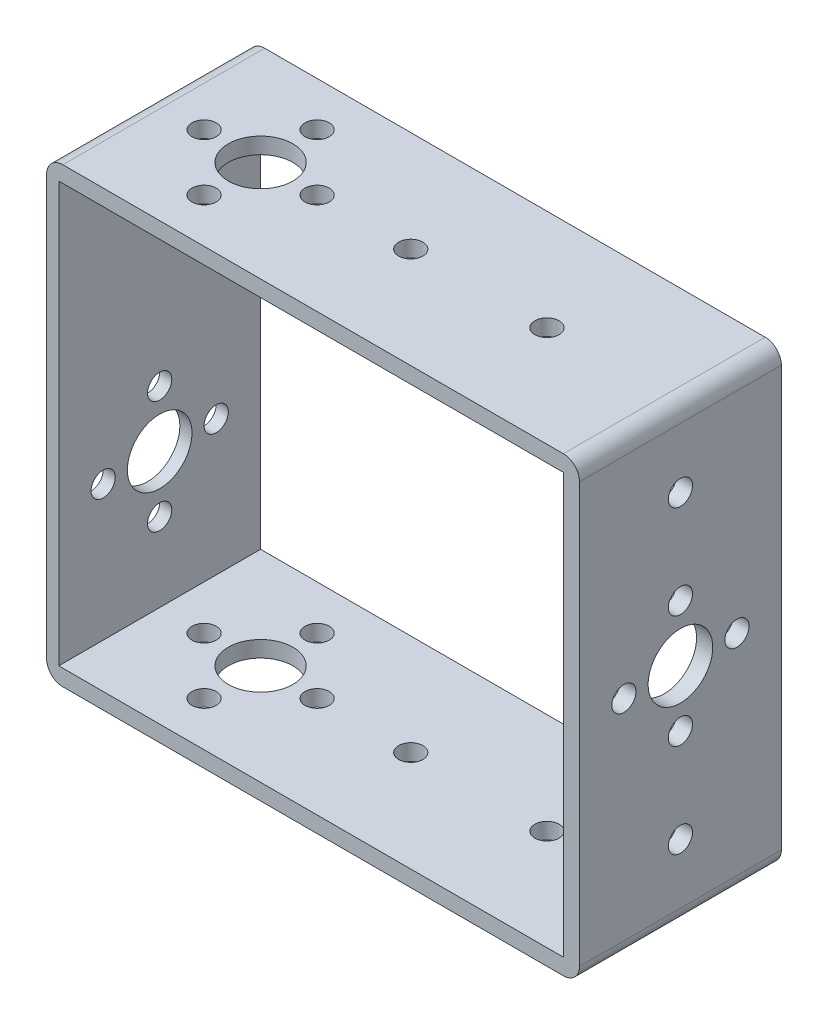
from build123d import *

# Parameters (mm, degrees)
SKETCH1_W                       = 64.5
SKETCH1_H                       = 56
BOSS_EXTRUDE1_DEPTH             = 25
CUT_EXTRUDE1_REACH              = 51.488
SKETCH2_W                       = 62.5
SKETCH2_H                       = 52
CUT_EXTRUDE2_REACH              = 76.627
SKETCH3_R                       = 4
SKETCH3_R_2                     = 1.5
CUT_EXTRUDE3_REACH              = 71.29
SKETCH4_R                       = 4
SKETCH4_R_2                     = 1.5
FILLET3_R                       = 2
BOSS_EXTRUDE2_REACH             = 51.488
SKETCH5_W                       = 1.5
SKETCH5_H                       = 25
BOSS_EXTRUDE2_DIRECTION_2_REACH = 51.488
FILLET4_R                       = 2
SKETCH6_R                       = 1.5
SKETCH6_R_2                     = 4
CUT_EXTRUDE5_DEPTH              = 1.5


with BuildPart() as part:
    # Sketch1 → Boss-Extrude1 (new body)
    with BuildSketch(Plane.XY):
        Rectangle(SKETCH1_W, SKETCH1_H)
    extrude(amount=BOSS_EXTRUDE1_DEPTH)

    # Sketch2 → Cut-Extrude1 (cut, up to next)
    with BuildSketch(Plane.XY.offset(25), mode=Mode.PRIVATE) as cut_extrude1_sk1:
        with Locations((-1, 0)):
            Rectangle(SKETCH2_W, SKETCH2_H)
    cut_extrude1_tool1 = extrude(cut_extrude1_sk1.sketch, amount=-CUT_EXTRUDE1_REACH, mode=Mode.PRIVATE) & part.part
    add(cut_extrude1_tool1.solids().sort_by_distance((-1, 0, 25))[0], mode=Mode.SUBTRACT)

    # Sketch3 → Cut-Extrude2 (cut, up to next)
    with BuildSketch(Plane(origin=(32.25, 0, 0), x_dir=(0, 0, -1), z_dir=(1, 0, 0)), mode=Mode.PRIVATE) as cut_extrude2_sk1:
        with Locations((-12.5, 0)):
            Circle(SKETCH3_R)
    cut_extrude2_tool1 = extrude(cut_extrude2_sk1.sketch, amount=-CUT_EXTRUDE2_REACH, mode=Mode.PRIVATE) & part.part
    # Sketch3 → Cut-Extrude2 (cut, up to next)
    with BuildSketch(Plane(origin=(32.25, 0, 0), x_dir=(0, 0, -1), z_dir=(1, 0, 0)), mode=Mode.PRIVATE) as cut_extrude2_sk2:
        with Locations((-5.5, 0)):
            Circle(SKETCH3_R_2)
    cut_extrude2_tool2 = extrude(cut_extrude2_sk2.sketch, amount=-CUT_EXTRUDE2_REACH, mode=Mode.PRIVATE) & part.part
    # Sketch3 → Cut-Extrude2 (cut, up to next)
    with BuildSketch(Plane(origin=(32.25, 0, 0), x_dir=(0, 0, -1), z_dir=(1, 0, 0)), mode=Mode.PRIVATE) as cut_extrude2_sk3:
        with Locations((-12.5, 18.6)):
            Circle(SKETCH3_R_2)
    cut_extrude2_tool3 = extrude(cut_extrude2_sk3.sketch, amount=-CUT_EXTRUDE2_REACH, mode=Mode.PRIVATE) & part.part
    # Sketch3 → Cut-Extrude2 (cut, up to next)
    with BuildSketch(Plane(origin=(32.25, 0, 0), x_dir=(0, 0, -1), z_dir=(1, 0, 0)), mode=Mode.PRIVATE) as cut_extrude2_sk4:
        with Locations((-12.5, -7)):
            Circle(SKETCH3_R_2)
    cut_extrude2_tool4 = extrude(cut_extrude2_sk4.sketch, amount=-CUT_EXTRUDE2_REACH, mode=Mode.PRIVATE) & part.part
    # Sketch3 → Cut-Extrude2 (cut, up to next)
    with BuildSketch(Plane(origin=(32.25, 0, 0), x_dir=(0, 0, -1), z_dir=(1, 0, 0)), mode=Mode.PRIVATE) as cut_extrude2_sk5:
        with Locations((-19.5, 0)):
            Circle(SKETCH3_R_2)
    cut_extrude2_tool5 = extrude(cut_extrude2_sk5.sketch, amount=-CUT_EXTRUDE2_REACH, mode=Mode.PRIVATE) & part.part
    # Sketch3 → Cut-Extrude2 (cut, up to next)
    with BuildSketch(Plane(origin=(32.25, 0, 0), x_dir=(0, 0, -1), z_dir=(1, 0, 0)), mode=Mode.PRIVATE) as cut_extrude2_sk6:
        with Locations((-12.5, 7)):
            Circle(SKETCH3_R_2)
    cut_extrude2_tool6 = extrude(cut_extrude2_sk6.sketch, amount=-CUT_EXTRUDE2_REACH, mode=Mode.PRIVATE) & part.part
    # Sketch3 → Cut-Extrude2 (cut, up to next)
    with BuildSketch(Plane(origin=(32.25, 0, 0), x_dir=(0, 0, -1), z_dir=(1, 0, 0)), mode=Mode.PRIVATE) as cut_extrude2_sk7:
        with Locations(Location((-12.5, -18.6, 0), (0, 0, 90))):
            Circle(SKETCH3_R_2)
    cut_extrude2_tool7 = extrude(cut_extrude2_sk7.sketch, amount=-CUT_EXTRUDE2_REACH, mode=Mode.PRIVATE) & part.part
    add(cut_extrude2_tool1.solids().sort_by_distance((32.25, 0, 12.5))[0], mode=Mode.SUBTRACT)
    add(cut_extrude2_tool2.solids().sort_by_distance((32.25, 0, 5.5))[0], mode=Mode.SUBTRACT)
    add(cut_extrude2_tool3.solids().sort_by_distance((32.25, 18.6, 12.5))[0], mode=Mode.SUBTRACT)
    add(cut_extrude2_tool4.solids().sort_by_distance((32.25, -7, 12.5))[0], mode=Mode.SUBTRACT)
    add(cut_extrude2_tool5.solids().sort_by_distance((32.25, 0, 19.5))[0], mode=Mode.SUBTRACT)
    add(cut_extrude2_tool6.solids().sort_by_distance((32.25, 7, 12.5))[0], mode=Mode.SUBTRACT)
    add(cut_extrude2_tool7.solids().sort_by_distance((32.25, -18.6, 12.5))[0], mode=Mode.SUBTRACT)

    # Sketch4 → Cut-Extrude3 (cut, up to next)
    with BuildSketch(Plane.XZ.offset(28), mode=Mode.PRIVATE) as cut_extrude3_sk1:
        with Locations(Location((-19.75, 12.5, 0), (0, 0, 270))):
            Circle(SKETCH4_R)
    cut_extrude3_tool1 = extrude(cut_extrude3_sk1.sketch, amount=-CUT_EXTRUDE3_REACH, mode=Mode.PRIVATE) & part.part
    # Sketch4 → Cut-Extrude3 (cut, up to next)
    with BuildSketch(Plane.XZ.offset(28), mode=Mode.PRIVATE) as cut_extrude3_sk2:
        with Locations(Location((-12.75, 12.5, 0), (0, 0, 270))):
            Circle(SKETCH4_R_2)
    cut_extrude3_tool2 = extrude(cut_extrude3_sk2.sketch, amount=-CUT_EXTRUDE3_REACH, mode=Mode.PRIVATE) & part.part
    # Sketch4 → Cut-Extrude3 (cut, up to next)
    with BuildSketch(Plane.XZ.offset(28), mode=Mode.PRIVATE) as cut_extrude3_sk3:
        with Locations(Location((-1.15, 12.5, 0), (0, 0, 270))):
            Circle(SKETCH4_R_2)
    cut_extrude3_tool3 = extrude(cut_extrude3_sk3.sketch, amount=-CUT_EXTRUDE3_REACH, mode=Mode.PRIVATE) & part.part
    # Sketch4 → Cut-Extrude3 (cut, up to next)
    with BuildSketch(Plane.XZ.offset(28), mode=Mode.PRIVATE) as cut_extrude3_sk4:
        with Locations(Location((15.72, 12.5, 0), (0, 0, 270))):
            Circle(SKETCH4_R_2)
    cut_extrude3_tool4 = extrude(cut_extrude3_sk4.sketch, amount=-CUT_EXTRUDE3_REACH, mode=Mode.PRIVATE) & part.part
    # Sketch4 → Cut-Extrude3 (cut, up to next)
    with BuildSketch(Plane.XZ.offset(28), mode=Mode.PRIVATE) as cut_extrude3_sk5:
        with Locations(Location((-19.75, 5.5, 0), (0, 0, 270))):
            Circle(SKETCH4_R_2)
    cut_extrude3_tool5 = extrude(cut_extrude3_sk5.sketch, amount=-CUT_EXTRUDE3_REACH, mode=Mode.PRIVATE) & part.part
    # Sketch4 → Cut-Extrude3 (cut, up to next)
    with BuildSketch(Plane.XZ.offset(28), mode=Mode.PRIVATE) as cut_extrude3_sk6:
        with Locations(Location((-26.75, 12.5, 0), (0, 0, 270))):
            Circle(SKETCH4_R_2)
    cut_extrude3_tool6 = extrude(cut_extrude3_sk6.sketch, amount=-CUT_EXTRUDE3_REACH, mode=Mode.PRIVATE) & part.part
    # Sketch4 → Cut-Extrude3 (cut, up to next)
    with BuildSketch(Plane.XZ.offset(28), mode=Mode.PRIVATE) as cut_extrude3_sk7:
        with Locations(Location((-19.75, 19.5, 0), (0, 0, 270))):
            Circle(SKETCH4_R_2)
    cut_extrude3_tool7 = extrude(cut_extrude3_sk7.sketch, amount=-CUT_EXTRUDE3_REACH, mode=Mode.PRIVATE) & part.part
    cut_extrude3_1 = cut_extrude3_tool1.solids().sort_by_distance((-19.75, -28, 12.5))[0]
    add(cut_extrude3_1, mode=Mode.SUBTRACT)
    cut_extrude3_2 = cut_extrude3_tool2.solids().sort_by_distance((-12.75, -28, 12.5))[0]
    add(cut_extrude3_2, mode=Mode.SUBTRACT)
    cut_extrude3_3 = cut_extrude3_tool3.solids().sort_by_distance((-1.15, -28, 12.5))[0]
    add(cut_extrude3_3, mode=Mode.SUBTRACT)
    cut_extrude3_4 = cut_extrude3_tool4.solids().sort_by_distance((15.72, -28, 12.5))[0]
    add(cut_extrude3_4, mode=Mode.SUBTRACT)
    cut_extrude3_5 = cut_extrude3_tool5.solids().sort_by_distance((-19.75, -28, 5.5))[0]
    add(cut_extrude3_5, mode=Mode.SUBTRACT)
    cut_extrude3_6 = cut_extrude3_tool6.solids().sort_by_distance((-26.75, -28, 12.5))[0]
    add(cut_extrude3_6, mode=Mode.SUBTRACT)
    cut_extrude3_7 = cut_extrude3_tool7.solids().sort_by_distance((-19.75, -28, 19.5))[0]
    add(cut_extrude3_7, mode=Mode.SUBTRACT)
    cut_extrude3 = cut_extrude3_1 + cut_extrude3_2 + cut_extrude3_3 + cut_extrude3_4 + cut_extrude3_5 + cut_extrude3_6 + cut_extrude3_7  # Cut-Extrude3 as one shape, for the pattern or mirror that repeats it

    # Mirror1: Cut-Extrude3 across plane
    add(cut_extrude3.mirror(Plane.ZX), mode=Mode.SUBTRACT)

    # Fillet3
    fillet3_edges = [part.edges().sort_by_distance(p)[0] for p in [
        (32.25, -28, 12.5),
        (32.25, 28, 12.5),
    ]]
    fillet(fillet3_edges, radius=FILLET3_R)

    # Boss-Extrude2: up to this face of the body (flat: up to its plane)
    boss_extrude2_end = Plane(part.part.faces().sort_by_distance((-1, 28, 0.673145601))[0])
    # Sketch5 → Boss-Extrude2 (add, up to the picked face)
    with BuildSketch(Plane(origin=(0, 0, 0), x_dir=(1, 0, 0), z_dir=(0, 1, 0)), mode=Mode.PRIVATE) as boss_extrude2_sk1:
        with Locations((-33, -12.5)):
            Rectangle(SKETCH5_W, SKETCH5_H)
    boss_extrude2_tool1 = split(extrude(boss_extrude2_sk1.sketch, amount=BOSS_EXTRUDE2_REACH, mode=Mode.PRIVATE), bisect_by=boss_extrude2_end, keep=Keep.BOTH, mode=Mode.PRIVATE)
    add(boss_extrude2_tool1.solids().sort_by(Axis((-33, 0, 12.5), (0, 1, 0)))[0])

    # Boss-Extrude2 direction 2: up to this face of the body (flat: up to its plane)
    boss_extrude2_direction_2_end = Plane(part.part.faces().sort_by_distance((-1, -28, 0.673145601))[0])
    # Sketch5 → Boss-Extrude2 direction 2 (add, up to the picked face)
    with BuildSketch(Plane(origin=(0, 0, 0), x_dir=(1, 0, 0), z_dir=(0, 1, 0)), mode=Mode.PRIVATE) as boss_extrude2_direction_2_sk1:
        with Locations((-33, -12.5)):
            Rectangle(SKETCH5_W, SKETCH5_H)
    boss_extrude2_direction_2_tool1 = split(extrude(boss_extrude2_direction_2_sk1.sketch, amount=-BOSS_EXTRUDE2_DIRECTION_2_REACH, mode=Mode.PRIVATE), bisect_by=boss_extrude2_direction_2_end, keep=Keep.BOTH, mode=Mode.PRIVATE)
    add(boss_extrude2_direction_2_tool1.solids().sort_by(Axis((-33, 0, 12.5), (0, -1, 0)))[0])

    # Fillet4
    fillet4_edges = [part.edges().sort_by_distance(p)[0] for p in [
        (-33.75, 28, 12.5),
        (-33.75, -28, 12.5),
    ]]
    fillet(fillet4_edges, radius=FILLET4_R)

    # Sketch6 → Cut-Extrude5 (cut)
    with BuildSketch(Plane(origin=(-32.25, 0, 0), x_dir=(0, 0, -1), z_dir=(1, 0, 0))):
        with Locations((-12.5, -2.25)):
            Circle(SKETCH6_R)
        with Locations((-19.5, -9.25)):
            Circle(SKETCH6_R)
        with Locations((-5.5, -9.25)):
            Circle(SKETCH6_R)
        with Locations((-12.5, -16.25)):
            Circle(SKETCH6_R)
        with Locations((-12.5, -9.25)):
            Circle(SKETCH6_R_2)
    extrude(amount=-CUT_EXTRUDE5_DEPTH, mode=Mode.SUBTRACT)


solid = part.part
